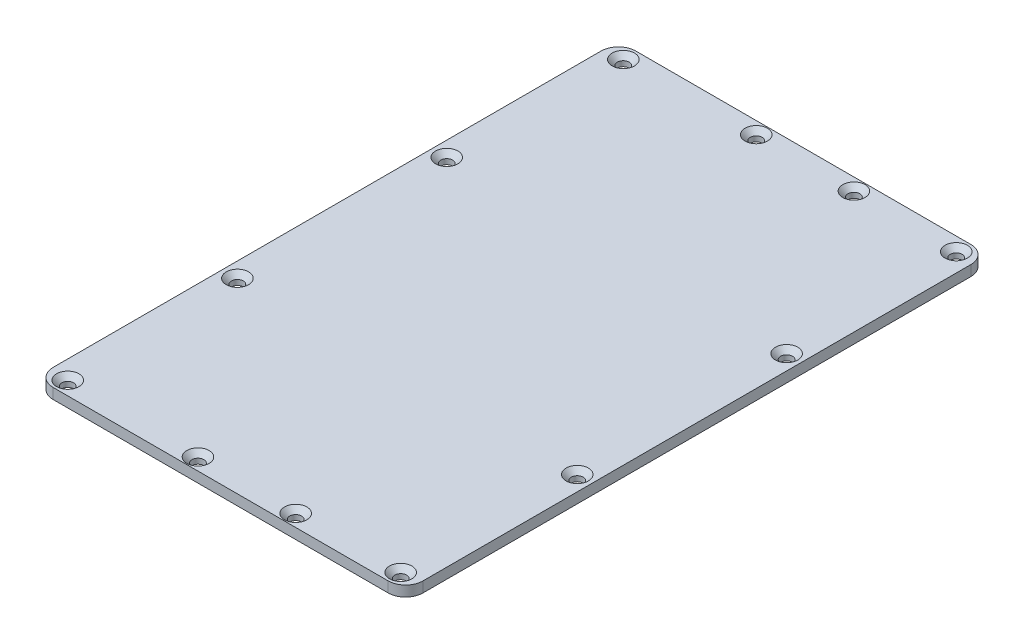
SolidWorks part; units mm, degrees
ref_plane "Front Plane" through (0, 0, 0) normal (0, 0, 1) x (1, 0, 0)
ref_plane "Top Plane" through (0, 0, 0) normal (0, 1, 0) x (1, 0, 0)
ref_plane "Right Plane" through (0, 0, 0) normal (1, 0, 0) x (0, 0, -1)
sketch "Sketch1" plane through (0, 0, 0) normal (0, 1, 0) x (1, 0, 0)
  line L8 (84.6562, 11.009) -> (84.6562, 168.009)
  line L9 (79.6562, 173.009) -> (-16.3438, 173.009)
  line L10 (-21.3438, 168.009) -> (-21.3438, 11.009)
  line L11 (-16.3438, 6.009) -> (79.6562, 6.009)
  line L12 (84.6562, 11.009) -> (84.6562, 168.009)
  line L13 (79.6562, 173.009) -> (-16.3438, 173.009)
  line L14 (-21.3438, 168.009) -> (-21.3438, 11.009)
  line L15 (-16.3438, 6.009) -> (79.6562, 6.009)
  arc A4 (84.6562, 168.009) -> (79.6562, 173.009) centre (79.6562, 168.009) ccw
  arc A5 (-16.3438, 173.009) -> (-21.3438, 168.009) centre (-16.3438, 168.009) ccw
  arc A6 (-21.3438, 11.009) -> (-16.3438, 6.009) centre (-16.3438, 11.009) ccw
  arc A7 (79.6562, 6.009) -> (84.6562, 11.009) centre (79.6562, 11.009) ccw
  arc A8 (84.6562, 168.009) -> (79.6562, 173.009) centre (79.6562, 168.009) ccw
  arc A9 (-16.3438, 173.009) -> (-21.3438, 168.009) centre (-16.3438, 168.009) ccw
  arc A10 (-21.3438, 11.009) -> (-16.3438, 6.009) centre (-16.3438, 11.009) ccw
  arc A11 (79.6562, 6.009) -> (84.6562, 11.009) centre (79.6562, 11.009) ccw
  point P0 (0, 0)
  dimension "D1" = 0
extrude "Boss-Extrude1" add sketch "Sketch1" along normal blind 3
hole_wizard "Hole size for slotted countersunk head screw type 0" positions "Sketch2" profile "Sketch3" countersink size "M3" standard "GB"
sketch "Sketch2" plane through (0, 3, 0) normal (0, 1, 0) x (1, 0, 0)
  point P0 (-16.0525, 169.1178)
  point P9 (79.365, 169.1178)
  point P12 (80.3562, 119.509)
  point P15 (80.3562, 59.509)
  point P18 (79.365, 9.9003)
  point P27 (-16.0525, 9.9003)
  point P30 (-17.0438, 59.509)
  point P33 (-17.0438, 119.509)
  point P42 (21.6562, 169.509)
  point P44 (49.6562, 169.509)
  point P46 (21.6562, 9.509)
  point P48 (49.6562, 9.509)
sketch "Sketch3" plane through (-16.0525, 3, -169.1178) normal (1, 0, 0) x (0, 0, 1)
  line L0 (0, 0) -> (0, 14.5215)
  line L1 (0, 14.5215) -> (1.7, 13.5)
  line L2 (1.7, 13.5) -> (1.7, 1.5)
  line L3 (1.7, 1.5) -> (3.2, 0)
  line L5 (3.2, 0) -> (0, 0)
  line L6 (-1.7, 1.5) -> (-3.2, 0) construction
  line L10 (0, 14.5215) -> (-1.7, 13.5) construction
  line L11 (0, -6.35) -> (0, 107.95) construction
  dimension "孔直径" = 3.4
  dimension "孔深度" = 13.5
  dimension "近端锥形沉头孔直径" = 6.4
  dimension "近端锥形沉头孔角度" = 90
  dimension "导头角度" = 118
